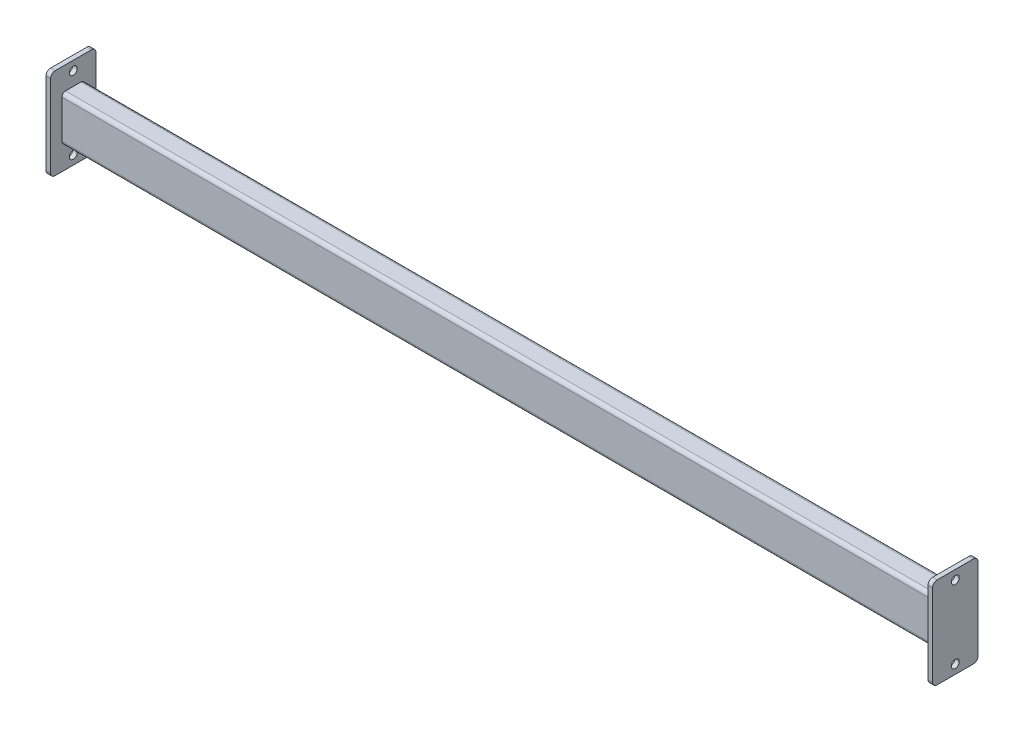
from build123d import *

# Parameters (mm, degrees)
GB_6728_1986_RECTANGULAR_HOLLOW_SECTION_DEPTH = 1930
SKETCH4_W                                     = 100
SKETCH4_H                                     = 200
BOSS_EXTRUDE1_DEPTH                           = 10
FILLET1_R                                     = 10
SKETCH9_W                                     = 8.75
SKETCH9_H                                     = 1950
M16_CLEARANCE_HOLE2_AT_2_COUNT                = 2
M16_CLEARANCE_HOLE2_AT_2_PITCH                = 160


with BuildPart() as part:
    # Sketch1 → Gb／6728-1986 rectangular hollow section 100 X 50 X 4 (1) (new body)
    with BuildSketch(Plane(origin=(-965, 0, 0), x_dir=(0, 0, -1), z_dir=(1, 0, 0))):
        with BuildLine():
            Line((-17, -50), (17, -50))
            ThreePointArc((17, -50), (22.656854249, -47.656854249), (25, -42))
            Line((25, -42), (25, 42))
            ThreePointArc((25, 42), (22.656854249, 47.656854249), (17, 50))
            Line((17, 50), (-17, 50))
            ThreePointArc((-17, 50), (-22.656854249, 47.656854249), (-25, 42))
            Line((-25, 42), (-25, -42))
            ThreePointArc((-25, -42), (-22.656854249, -47.656854249), (-17, -50))
        make_face()
        with BuildLine():
            Line((-17, -46), (17, -46))
            ThreePointArc((17, -46), (19.828427125, -44.828427125), (21, -42))
            Line((21, -42), (21, 42))
            ThreePointArc((21, 42), (19.828427125, 44.828427125), (17, 46))
            Line((17, 46), (-17, 46))
            ThreePointArc((-17, 46), (-19.828427125, 44.828427125), (-21, 42))
            Line((-21, 42), (-21, -42))
            ThreePointArc((-21, -42), (-19.828427125, -44.828427125), (-17, -46))
        make_face(mode=Mode.SUBTRACT)
    extrude(amount=GB_6728_1986_RECTANGULAR_HOLLOW_SECTION_DEPTH)


with BuildPart() as body_2:
    # Sketch4 → Boss-Extrude1 (new body)
    with BuildSketch(Plane.ZY.offset(965)):
        Rectangle(SKETCH4_W, SKETCH4_H)
    extrude(amount=BOSS_EXTRUDE1_DEPTH)

    # Fillet1
    fillet1_edges = [body_2.edges().sort_by_distance(p)[0] for p in [
        (-970, -100, 50),
        (-970, -100, -50),
        (-970, 100, -50),
        (-970, 100, 50),
    ]]
    fillet(fillet1_edges, radius=FILLET1_R)


with BuildPart() as body_3:
    # Mirror2: mirrored copy
    add(body_2.part.mirror(Plane.ZY))


with BuildPart() as m16_clearance_hole2_tool:
    # Sketch9 → M16 Clearance Hole2 (revolve)
    with BuildSketch(Plane(origin=(-975, 80, 0), x_dir=(0, 0, 1), z_dir=(0, 1, 0))):
        with Locations((4.375, 975)):
            Rectangle(SKETCH9_W, SKETCH9_H)
    m16_clearance_hole2 = revolve(axis=Axis((-981.35, 80, 0), (1, 0, 0)))


with BuildPart() as body_2_1:
    add(body_2.part)

    # M16 Clearance Hole2: cut by m16_clearance_hole2_tool
    add(m16_clearance_hole2_tool.part, mode=Mode.SUBTRACT)


with BuildPart() as body_3_1:
    add(body_3.part)

    # M16 Clearance Hole2: cut by m16_clearance_hole2_tool
    add(m16_clearance_hole2_tool.part, mode=Mode.SUBTRACT)


with BuildPart() as m16_clearance_hole2_at_2_tool:
    # M16 Clearance Hole2 at 2: M16 Clearance Hole2 ×2
    with Locations(*[(0, -i * M16_CLEARANCE_HOLE2_AT_2_PITCH, 0) for i in range(1, M16_CLEARANCE_HOLE2_AT_2_COUNT)]):
        add(m16_clearance_hole2)


with BuildPart() as body_2_2:
    add(body_2_1.part)

    # M16 Clearance Hole2 at 2: cut by m16_clearance_hole2_at_2_tool
    add(m16_clearance_hole2_at_2_tool.part, mode=Mode.SUBTRACT)


with BuildPart() as body_3_2:
    add(body_3_1.part)

    # M16 Clearance Hole2 at 2: cut by m16_clearance_hole2_at_2_tool
    add(m16_clearance_hole2_at_2_tool.part, mode=Mode.SUBTRACT)


solid = Compound([part.part, body_2_2.part, body_3_2.part])
